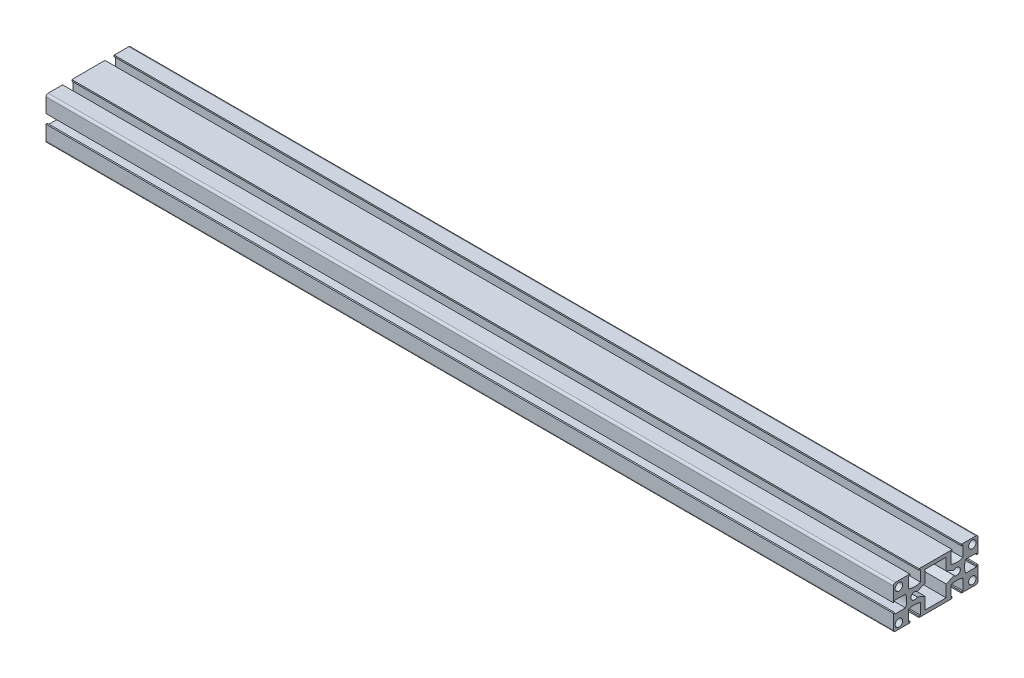
from build123d import *

# Parameters (mm, degrees)
SKETCH1_R                 = 2.65
F_30_X_60G_X_R1_5_1_DEPTH = 600


with BuildPart() as part:
    # Sketch1 → 工业铝型材 30 X 60G X R1.5(1) (new body)
    with BuildSketch(Plane.YZ.offset(-300)):
        with BuildLine():
            Line((-3.25, 30), (-3.25, 29))
            Line((-3.25, 29), (-4.25, 29))
            Line((-4.25, 29), (-4.25, 21.277812156))
            ThreePointArc((-4.25, 21.277812156), (0, 20.5), (4.25, 21.277812156))
            Line((4.25, 21.277812156), (4.25, 29))
            Line((4.25, 29), (3.25, 29))
            Line((3.25, 29), (3.25, 30))
            Line((3.25, 30), (13.5, 30))
            ThreePointArc((13.5, 30), (14.560660172, 29.560660172), (15, 28.5))
            Line((15, 28.5), (15, 18.25))
            Line((15, 18.25), (14, 18.25))
            Line((14, 18.25), (14, 19.25))
            Line((14, 19.25), (6.277812156, 19.25))
            ThreePointArc((6.277812156, 19.25), (5.5, 15), (6.277812156, 10.75))
            Line((6.277812156, 10.75), (14, 10.75))
            Line((14, 10.75), (14, 11.75))
            Line((14, 11.75), (15, 11.75))
            Line((15, 11.75), (15, -11.75))
            Line((15, -11.75), (14, -11.75))
            Line((14, -11.75), (14, -10.75))
            Line((14, -10.75), (6.277812156, -10.75))
            ThreePointArc((6.277812156, -10.75), (5.5, -15), (6.277812156, -19.25))
            Line((6.277812156, -19.25), (14, -19.25))
            Line((14, -19.25), (14, -18.25))
            Line((14, -18.25), (15, -18.25))
            Line((15, -18.25), (15, -28.5))
            ThreePointArc((15, -28.5), (14.560660172, -29.560660172), (13.5, -30))
            Line((13.5, -30), (3.25, -30))
            Line((3.25, -30), (3.25, -29))
            Line((3.25, -29), (4.25, -29))
            Line((4.25, -29), (4.25, -21.277812156))
            ThreePointArc((4.25, -21.277812156), (0, -20.5), (-4.25, -21.277812156))
            Line((-4.25, -21.277812156), (-4.25, -29))
            Line((-4.25, -29), (-3.25, -29))
            Line((-3.25, -29), (-3.25, -30))
            Line((-3.25, -30), (-13.5, -30))
            ThreePointArc((-13.5, -30), (-14.560660172, -29.560660172), (-15, -28.5))
            Line((-15, -28.5), (-15, -18.25))
            Line((-15, -18.25), (-14, -18.25))
            Line((-14, -18.25), (-14, -19.25))
            Line((-14, -19.25), (-6.277812156, -19.25))
            ThreePointArc((-6.277812156, -19.25), (-5.5, -15), (-6.277812156, -10.75))
            Line((-6.277812156, -10.75), (-14, -10.75))
            Line((-14, -10.75), (-14, -11.75))
            Line((-14, -11.75), (-15, -11.75))
            Line((-15, -11.75), (-15, 11.75))
            Line((-15, 11.75), (-14, 11.75))
            Line((-14, 11.75), (-14, 10.75))
            Line((-14, 10.75), (-6.277812156, 10.75))
            ThreePointArc((-6.277812156, 10.75), (-5.5, 15), (-6.277812156, 19.25))
            Line((-6.277812156, 19.25), (-14, 19.25))
            Line((-14, 19.25), (-14, 18.25))
            Line((-14, 18.25), (-15, 18.25))
            Line((-15, 18.25), (-15, 28.5))
            ThreePointArc((-15, 28.5), (-14.560660172, 29.560660172), (-13.5, 30))
            Line((-13.5, 30), (-3.25, 30))
        make_face()
        with Locations((-11, 26)):
            Circle(SKETCH1_R, mode=Mode.SUBTRACT)
        with Locations((11, 26)):
            Circle(SKETCH1_R, mode=Mode.SUBTRACT)
        with Locations((11, -26)):
            Circle(SKETCH1_R, mode=Mode.SUBTRACT)
        with Locations((-11, -26)):
            Circle(SKETCH1_R, mode=Mode.SUBTRACT)
        with BuildLine():
            Line((-12.5, 7.5), (-4, 7.5))
            Line((-4, 7.5), (-1.665625283, 13.135679101))
            ThreePointArc((-1.665625283, 13.135679101), (0, 17.5), (1.665625283, 13.135679101))
            Line((1.665625283, 13.135679101), (4, 7.5))
            Line((4, 7.5), (12.5, 7.5))
            Line((12.5, 7.5), (12.5, -7.5))
            Line((12.5, -7.5), (4, -7.5))
            Line((4, -7.5), (1.665625283, -13.135679101))
            ThreePointArc((1.665625283, -13.135679101), (0, -17.5), (-1.665625283, -13.135679101))
            Line((-1.665625283, -13.135679101), (-4, -7.5))
            Line((-4, -7.5), (-12.5, -7.5))
            Line((-12.5, -7.5), (-12.5, 7.5))
        make_face(mode=Mode.SUBTRACT)
    extrude(amount=F_30_X_60G_X_R1_5_1_DEPTH)


solid = part.part
